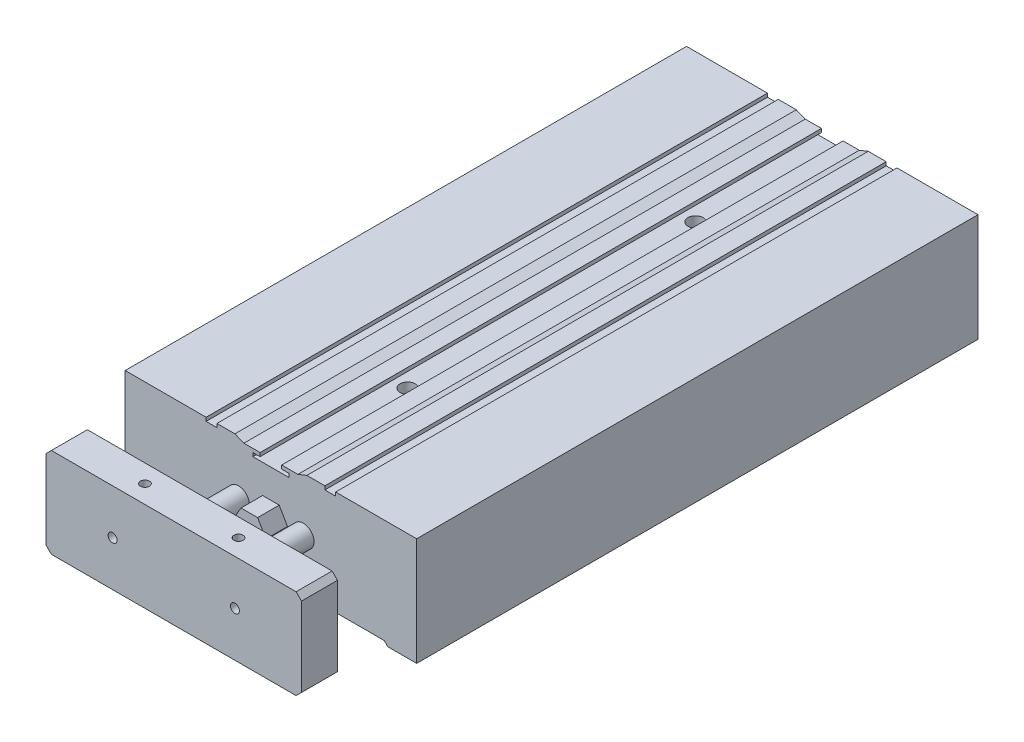
from build123d import *

# Parameters (mm, degrees)
EXTRUDE1_DEPTH             = 156
SKETCH2_R                  = 3
EXTRUDE2_DEPTH             = 17
EXTRUDE3_DEPTH             = 10
M3X0_5_TAPPED_HOLE1_D      = 2.5
M3X0_5_TAPPED_HOLE1_DEPTH  = 10
M3X0_5_TAPPED_HOLE2_D      = 2.5
SKETCH15_W                 = 10
SKETCH15_H                 = 10
EXTRUDE4_DEPTH             = 1
EXTRUDE5_DEPTH             = 6
SKETCH20_W                 = 2.1
SKETCH20_H                 = 30
M5_TAPPED_HOLE1_AT_2_COUNT = 2
M5_TAPPED_HOLE1_AT_2_PITCH = 80


with BuildPart() as part:
    # Sketch1 → Extrude1 (new body)
    with BuildSketch(Plane.XY):
        Polygon((0, 0), (8, 0), (9, 1), (33.5, 1), (34.5, 0), (46.5, 0), (47.5, 1), (72, 1), (73, 0), (81, 0), (81, 30), (58.5, 30), (58.5, 29), (55.5, 29), (55.5, 30), (50.5, 30), (48, 29), (43.5, 29), (43.5, 28), (45.5, 28), (45.5, 27), (35.5, 27), (35.5, 28), (37.5, 28), (37.5, 29), (33, 29), (30.5, 30), (25.5, 30), (25.5, 29), (22.5, 29), (22.5, 30), (0, 30), align=None)
    extrude(amount=EXTRUDE1_DEPTH)

    # Sketch2 → Extrude2 (add)
    with BuildSketch(Plane.XY.offset(156)):
        with Locations(Location((31.5, 15, 0), (0, 0, 180))):
            Circle(SKETCH2_R)
        with Locations(Location((49.5, 15, 0), (0, 0, 180))):
            Circle(SKETCH2_R)
    extrude(amount=EXTRUDE2_DEPTH)

    # Sketch3 → Extrude3 (add)
    with BuildSketch(Plane.XY.offset(173)):
        Polygon((6.5, 27.5), (74.5, 27.5), (76, 26), (76, 4), (74.5, 2.5), (6.5, 2.5), (5, 4), (5, 26), align=None)
    extrude(amount=EXTRUDE3_DEPTH)

    # M3x0.5 Tapped Hole1
    with Locations(Plane.XY.offset(183)):
        with Locations((23.5, 15), (57.5, 15)):
            Hole(M3X0_5_TAPPED_HOLE1_D / 2, depth=M3X0_5_TAPPED_HOLE1_DEPTH)

    # M3x0.5 Tapped Hole2 (through all)
    with Locations(Plane(origin=(0, 27.5, 0), x_dir=(-1, 0, 0), z_dir=(0, 1, 0))):
        with Locations((-27.5, 178), (-53.5, 178)):
            Hole(M3X0_5_TAPPED_HOLE2_D / 2)

    # Sketch15 → Extrude4 (add)
    with BuildSketch(Plane(origin=(0, 0, 173), x_dir=(-1, 0, 0), z_dir=(0, 0, -1))):
        with Locations((-40.5, 15)):
            Rectangle(SKETCH15_W, SKETCH15_H)
    extrude(amount=EXTRUDE4_DEPTH)

    # Sketch20 → M5 Tapped Hole1 (revolve, cut)
    with BuildSketch(Plane(origin=(40.5, 0, 118), x_dir=(0, 0, -1), z_dir=(1, 0, 0))):
        with Locations((1.05, 15)):
            Rectangle(SKETCH20_W, SKETCH20_H)
    m5_tapped_hole1 = revolve(axis=Axis((40.5, -6.35, 118), (0, 1, 0)), mode=Mode.SUBTRACT)

    # M5 Tapped Hole1 at 2: M5 Tapped Hole1 ×2
    with Locations(*[(0, 0, -i * M5_TAPPED_HOLE1_AT_2_PITCH) for i in range(1, M5_TAPPED_HOLE1_AT_2_COUNT)]):
        add(m5_tapped_hole1, mode=Mode.SUBTRACT)


with BuildPart() as body_2:
    # Sketch16 → Extrude5 (new body)
    with BuildSketch(Plane.XY.offset(156)):
        Polygon((42.809401077, 11), (45.118802154, 15), (42.809401077, 19), (38.190598923, 19), (35.881197846, 15), (38.190598923, 11), align=None)
    extrude(amount=EXTRUDE5_DEPTH)


solid = Compound([part.part, body_2.part])
